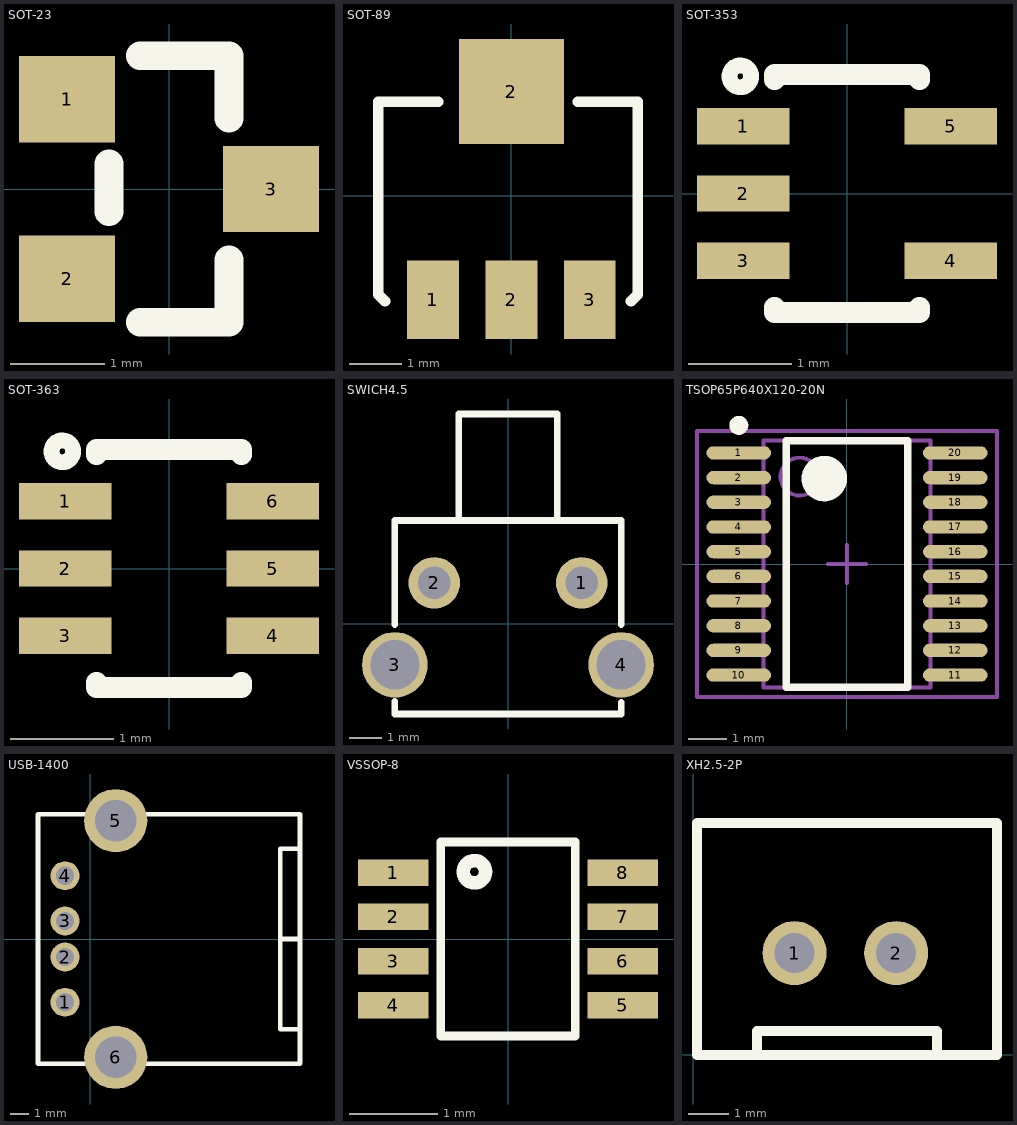
[diagram p0: the footprints below, top view; thin cyan lines are the x and y axes]
# Altium footprint library MISC84456-6.PcbLib: 41 footprints (part 3 of 3)
Each footprint in its own frame and in the unit in brackets; x right, y up, seen from the top. Pads: shape width x height; smd on the part's side, far side on the other; paste and mask are expansions set on the pad; w line width, h text height; cw(c..) or ccw(c..) is an arc to the next point about the centre after c.

## SOT-23 [mil]
height 374.02
pads (3):
  rect 40x36 smd: 1(-42.5,37.4) 2(-42.5,-37.4) 3(42.5,0)
Top Overlay:
  lines w12: -25,-9.5 -25,10.5 ; -12,-55.5 25,-55.5 25,-29.5 ; -12,55.5 25,55.5 25,29.5
3D body: height 39.37, standoff -0.79, extent -47,-56.98 50.48,57.98

## SOT-89 [mil]
height 47.24
pads (4):
  rect 39x59 smd: 1(-59,-78.3) 2(0,-78.3) 3(59,-78.3)
  rect 79x79 smd: 2(0,78.3)
Top Overlay:
  lines w8: -95,-79.3 -100,-74.3 -100,70.7 -55,70.7 ; 50,70.7 95,70.7 95,-74.3 90,-79.3

## SOT-353 [mm]
height 9.5
pads (5):
  rect 0.896x0.35 smd: 1(-1.002,0.65) 2(-1.002,0) 3(-1.002,-0.65) 4(1.002,-0.65) 5(1.002,0.65)
Top Overlay:
  circle w0.152: c-1.031,1.133 r0.105
  lines w0.2: -0.7,-1.1 -0.7,-1.15 0.7,-1.15 0.7,-1.1 ; -0.7,1.1 -0.7,1.15 0.7,1.15 0.7,1.1

## SOT-363 [mm]
height 1.016
pads (6):
  rect 0.896x0.35 smd: 1(-1.002,0.65) 2(-1.002,0) 3(-1.002,-0.65) 4(1.002,-0.65) 5(1.002,0) 6(1.002,0.65)
Top Overlay:
  circle w0.152: c-1.031,1.133 r0.105
  lines w0.2: -0.7,-1.1 -0.7,-1.15 0.7,-1.15 0.7,-1.1 ; -0.7,1.1 -0.7,1.15 0.7,1.15 0.7,1.1
3D body: height 1, standoff 0, extent -1.15,-1.041 1.15,1.059

## SWICH4.5 [mm] "6.6mm"
pads (4):
  round 1.575 hole 1: 1(2.25,1.25) 2(-2.25,1.25)
  round 2 hole 1.5: 3(-3.45,-1.25) 4(3.45,-1.25)
Top Overlay:
  lines w0.203: -3.45,-2.361 -3.45,-2.75 3.45,-2.75 3.45,-2.387 ; -3.45,-0.02 -3.45,3.15 3.454,3.15 3.454,-0.02 ; -1.5,3.15 -1.5,6.4 1.5,6.4 1.5,3.15

## TSOP65P640X120-20N [mm] "TSOP, 20-Leads, Body 6.5x4.4mm (max), Pitch 0.65"
height 1.2
pads (20):
  oval 1.7x0.35 smd: 1(-2.85,2.925) 2(-2.85,2.275) 3(-2.85,1.625) 4(-2.85,0.975) 5(-2.85,0.325) 6(-2.85,-0.325) 7(-2.85,-0.975) 8(-2.85,-1.625) 9(-2.85,-2.275) 10(-2.85,-2.925) 11(2.85,-2.925) 12(2.85,-2.275) 13(2.85,-1.625) 14(2.85,-0.975) 15(2.85,-0.325) 16(2.85,0.325) 17(2.85,0.975) 18(2.85,1.625) 19(2.85,2.275) 20(2.85,2.925)
Top Overlay:
  circle w0.6: c-0.6,2.25 r0.3
  circle w0.25: c-2.85,3.65 r0.125
  lines w0.2: -1.6,-3.25 1.6,-3.25 1.6,3.25 -1.6,3.25 -1.6,-3.25
Mechanical 13:
  circle w0.1: c-1.25,2.3 r0.5
  lines w0.1: -2.2,-3.25 2.2,-3.25 2.2,3.25 -2.2,3.25 -2.2,-3.25
Mechanical 15:
  lines w0.1: -0.5,0 0.5,0 ; 0,-0.5 0,0.5 ; -3.95,-3.5 3.95,-3.5 3.95,3.5 -3.95,3.5 -3.95,-3.5
3D body: height 1.2, standoff 0.09, extent -2.2,-3.25 2.2,3.25

## USB-1400 [mm] "5.5mm"
pads (6):
  round 1.6 hole 1: 1(-1.4,-3.5) 2(-1.4,-1) 3(-1.4,1) 4(-1.4,3.5)
  round 3.5 hole 2.3: 5(1.4,6.55) 6(1.4,-6.55)
Top Overlay:
  lines w0.254: 10.5,0 11.6,0 ; 11.5,-5 10.5,-5 10.5,5 11.6,5 ; -2.9,-6.9 11.6,-6.9 11.6,6.9 -2.9,6.9 -2.9,-6.9

## VSSOP-8 [mm]
height 3.98
pads (8):
  rect 0.8x0.3 smd: 1(-1.3,0.75) 2(-1.3,0.25) 3(-1.3,-0.25) 4(-1.3,-0.75) 5(1.3,-0.75) 6(1.3,-0.25) 7(1.3,0.25) 8(1.3,0.75)
Top Overlay:
  circle w0.152: c-0.381,0.762 r0.127
  lines w0.1: -0.762,-1.1 -0.762,1.1 0.762,1.1 0.762,-1.1 -0.762,-1.1

## XH2.5-2P [mm]
pads (2):
  round 1.6 hole 1: 1(2.54,2.54) 2(5.08,2.54)
Top Overlay:
  lines w0.254: 1.599,-0.007 1.599,0.593 6.1,0.593 6.1,0 ; 0.099,-0.007 7.6,-0.007 7.6,5.793 0.099,5.793 0.099,-0.007